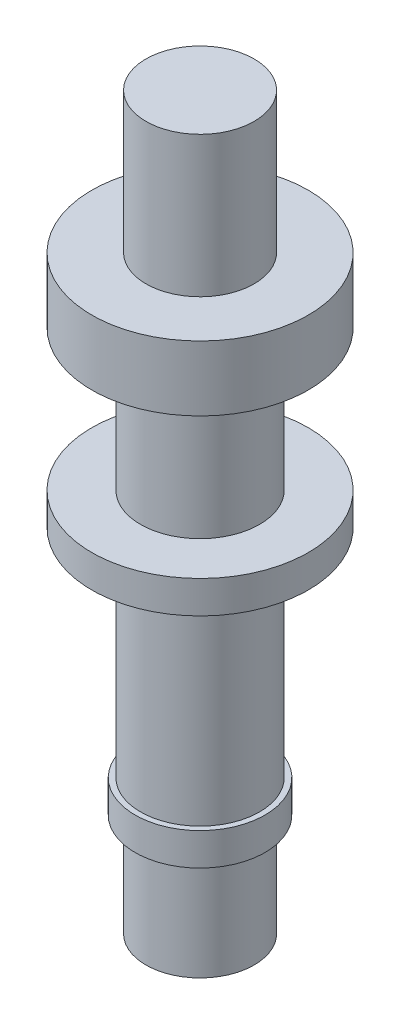
SolidWorks part; units mm, degrees
ref_plane "前视基准面" through (0, 0, 0) normal (0, 0, 1) x (1, 0, 0)
ref_plane "上视基准面" through (0, 0, 0) normal (0, 1, 0) x (1, 0, 0)
ref_plane "右视基准面" through (0, 0, 0) normal (1, 0, 0) x (0, 0, -1)
sketch "草图1" plane through (0, 0, 0) normal (0, 0, 1) x (1, 0, 0)
  line L0 (0, -28.7184) -> (0, 167.1112) construction
  line L1 (0, 0) -> (5, 0)
  line L2 (5, 0) -> (5, 9.5)
  line L3 (5, 9.5) -> (6, 9.5)
  line L4 (6, 9.5) -> (6, 12.5)
  line L5 (6, 12.5) -> (5.5, 12.5)
  line L6 (5.5, 12.5) -> (5.5, 32.5)
  line L7 (5.5, 32.5) -> (10, 32.5)
  line L8 (10, 32.5) -> (10, 35.5)
  line L9 (10, 35.5) -> (5.5, 35.5)
  line L10 (5.5, 35.5) -> (5.5, 48.5)
  line L11 (5.5, 48.5) -> (10, 48.5)
  line L12 (10, 48.5) -> (10, 54.5)
  line L13 (10, 54.5) -> (5, 54.5)
  line L14 (5, 54.5) -> (5, 67.5)
  line L15 (5, 67.5) -> (0, 67.5)
  line L16 (0, 0) -> (0, 67.5)
  dimension "D1" = 5
  dimension "D2" = 9.5
  dimension "D3" = 3
  dimension "D4" = 12
  dimension "D5" = 11
  dimension "D6" = 20
  dimension "D7" = 3
  dimension "D8" = 20
  dimension "D9" = 6
  dimension "D10" = 20
  dimension "D11" = 11
  dimension "D12" = 19
  dimension "D13" = 67.5
  dimension "D14" = 10
revolve "旋转1" add sketch "草图1" angle 360 about L0
